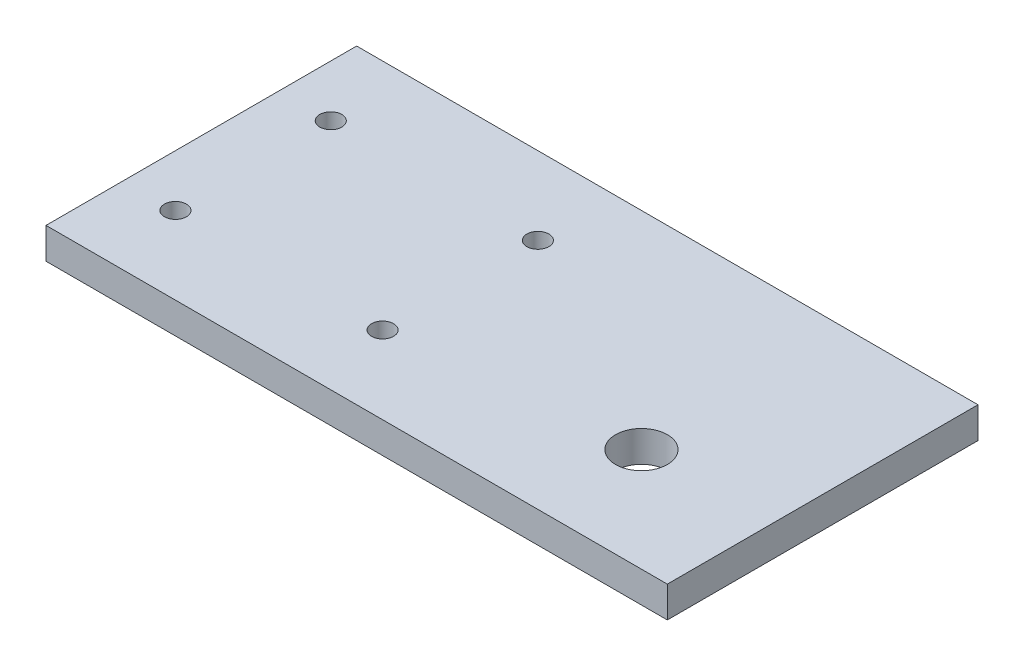
SolidWorks part; units mm, degrees
ref_plane "前视基准面" through (0, 0, 0) normal (0, 0, 1) x (1, 0, 0)
ref_plane "上视基准面" through (0, 0, 0) normal (0, 1, 0) x (1, 0, 0)
ref_plane "右视基准面" through (0, 0, 0) normal (1, 0, 0) x (0, 0, -1)
sketch "草图1" plane through (0, 0, 0) normal (0, 1, 0) x (1, 0, 0)
  line L1 (0, 0) -> (240, 0)
  line L2 (0, 0) -> (0, 120)
  line L3 (0, 120) -> (240, 120)
  line L4 (240, 0) -> (240, 120)
  line L5 (0, 0) -> (240, 120) construction
  line L6 (0, 120) -> (240, 0) construction
  circle A0 centre (20, 30) radius 4.25
  circle A1 centre (20, 90) radius 4.25
  circle A2 centre (100, 90) radius 4.25
  circle A3 centre (100, 30) radius 4.25
  circle A4 centre (190, 40) radius 10
  point P4 (120, 60)
  point P14 (0, 0)
  dimension "D3" = 60
  dimension "D5" = 20
  dimension "D7" = 8.5
  dimension "D8" = 8.5
  dimension "D9" = 20
  dimension "D10" = 90
  dimension "D1" = 240
  dimension "D2" = 120
  dimension "D4" = 30
  dimension "D6" = 80
  dimension "D11" = 80
extrude "凸台-拉伸1" add sketch "草图1" along normal blind 12 contours L3 L4 L1 L2
cosmetic thread "装饰螺纹线2"
cosmetic thread "装饰螺纹线3"
cosmetic thread "装饰螺纹线4"
cosmetic thread "装饰螺纹线5"
cosmetic thread "装饰螺纹线6"
